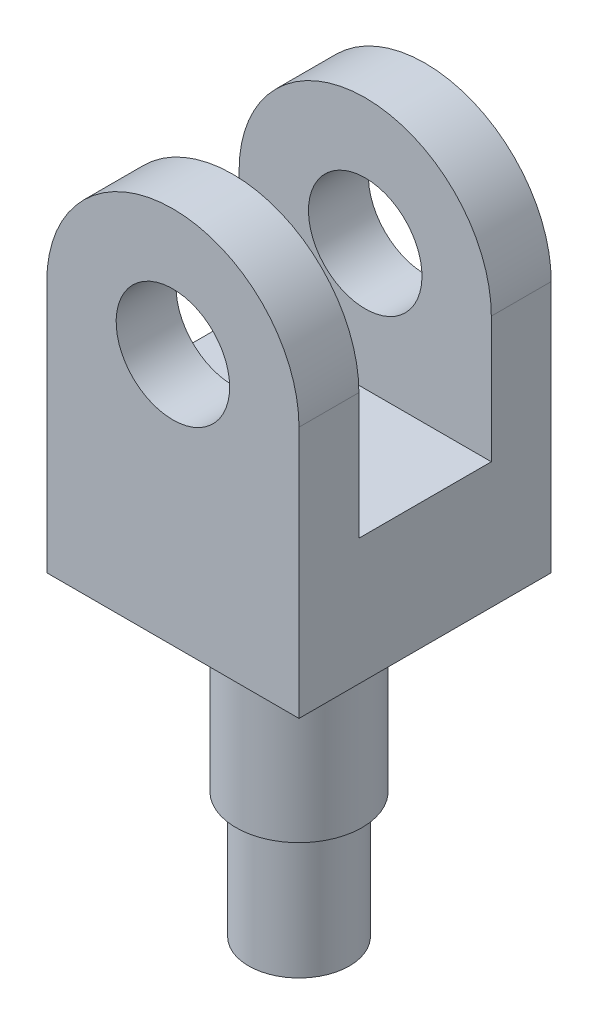
from build123d import *

# Parameters (mm, degrees)
SKETCH1_R           = 45
BOSS_EXTRUDE2_DEPTH = 200
SKETCH2_W           = 105
SKETCH2_H           = 318.049906591
CUT_EXTRUDE1_DEPTH  = 325.763563649
SKETCH3_R           = 50
BOSS_EXTRUDE3_DEPTH = 140
SKETCH4_R           = 50
BOSS_EXTRUDE4_DEPTH = 10
SKETCH5_R           = 40
BOSS_EXTRUDE5_DEPTH = 100


with BuildPart() as part:
    # Sketch1 → Boss-Extrude2 (new body)
    with BuildSketch(Plane.XY):
        with BuildLine():
            Line((140.402467833, -159.597532167), (-59.597532167, -159.597532167))
            Line((-59.597532167, -159.597532167), (-59.597532167, 40.402467833))
            ThreePointArc((-59.597532167, 40.402467833), (40.402467833, 140.402467833), (140.402467833, 40.402467833))
            Line((140.402467833, 40.402467833), (140.402467833, -159.597532167))
        make_face()
        with Locations((40.402467833, 40.402467833)):
            Circle(SKETCH1_R, mode=Mode.SUBTRACT)
    extrude(amount=BOSS_EXTRUDE2_DEPTH)

    # Sketch2 → Cut-Extrude1 (cut, through all)
    with BuildSketch(Plane(origin=(140.402467833, 0, 0), x_dir=(0, 0, -1), z_dir=(1, 0, 0))):
        with Locations((-100, 99.427421129)):
            Rectangle(SKETCH2_W, SKETCH2_H)
    extrude(amount=-CUT_EXTRUDE1_DEPTH, mode=Mode.SUBTRACT)

    # Sketch3 → Boss-Extrude3 (add)
    with BuildSketch(Plane.XZ.offset(159.597532167)):
        with Locations((40.402467833, 100)):
            Circle(SKETCH3_R)
    extrude(amount=BOSS_EXTRUDE3_DEPTH)

    # Sketch4 → Boss-Extrude4 (add)
    with BuildSketch(Plane.XZ.offset(299.597532167)):
        with Locations((40.402467833, 100)):
            Circle(SKETCH4_R)
    extrude(amount=BOSS_EXTRUDE4_DEPTH)

    # Sketch5 → Boss-Extrude5 (add)
    with BuildSketch(Plane.XZ.offset(309.597532167)):
        with Locations((40.402467833, 100)):
            Circle(SKETCH5_R)
    extrude(amount=BOSS_EXTRUDE5_DEPTH)


solid = part.part
